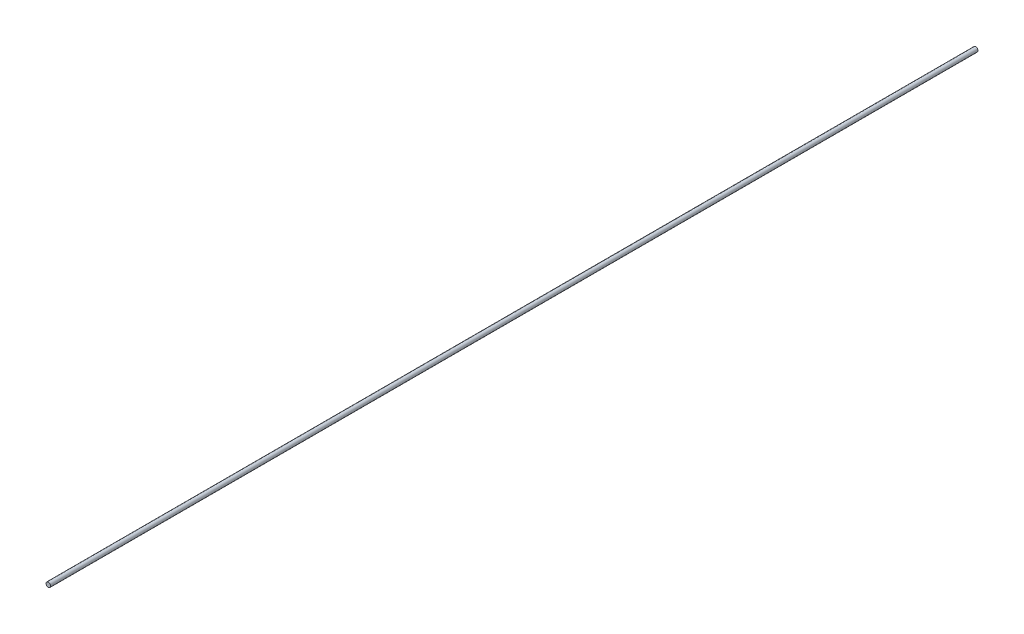
SolidWorks part; units mm, degrees
material "SWM-B"
ref_plane "Front Plane" through (0, 0, 0) normal (0, 0, 1) x (1, 0, 0)
ref_plane "Top Plane" through (0, 0, 0) normal (0, 1, 0) x (1, 0, 0)
ref_plane "Right Plane" through (0, 0, 0) normal (1, 0, 0) x (0, 0, -1)
sketch "Sketch2" plane through (0, 0, 0) normal (0, 0, 1) x (1, 0, 0)
  circle A0 centre (0, 0) radius 2
  dimension "D1" = 4
extrude "Boss-Extrude1" add sketch "Sketch2" along normal blind 810
